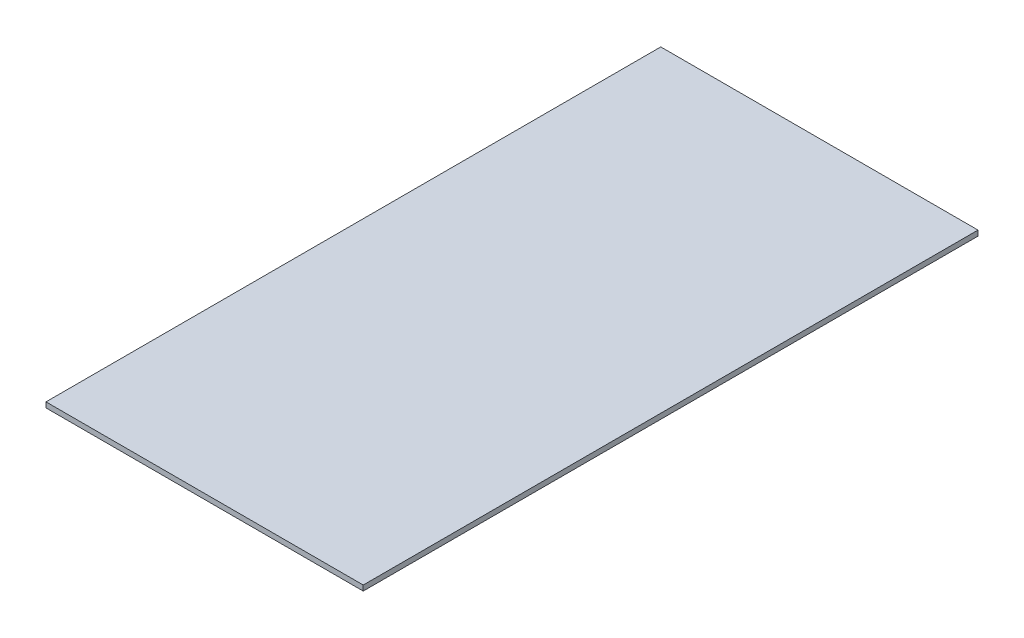
SolidWorks part; units mm, degrees
ref_plane "前视基准面" through (0, 0, 0) normal (0, 0, 1) x (1, 0, 0)
ref_plane "上视基准面" through (0, 0, 0) normal (0, 1, 0) x (1, 0, 0)
ref_plane "右视基准面" through (0, 0, 0) normal (1, 0, 0) x (0, 0, -1)
sketch "草图1" plane through (0, 0, 0) normal (0, 1, 0) x (1, 0, 0)
  line L0 (0, 0) -> (903, 0)
  line L1 (903, 0) -> (903, -1750)
  line L2 (903, -1750) -> (0, -1750)
  line L3 (0, -1750) -> (0, 0)
extrude "凸台-拉伸1" add sketch "草图1" along normal blind 15
